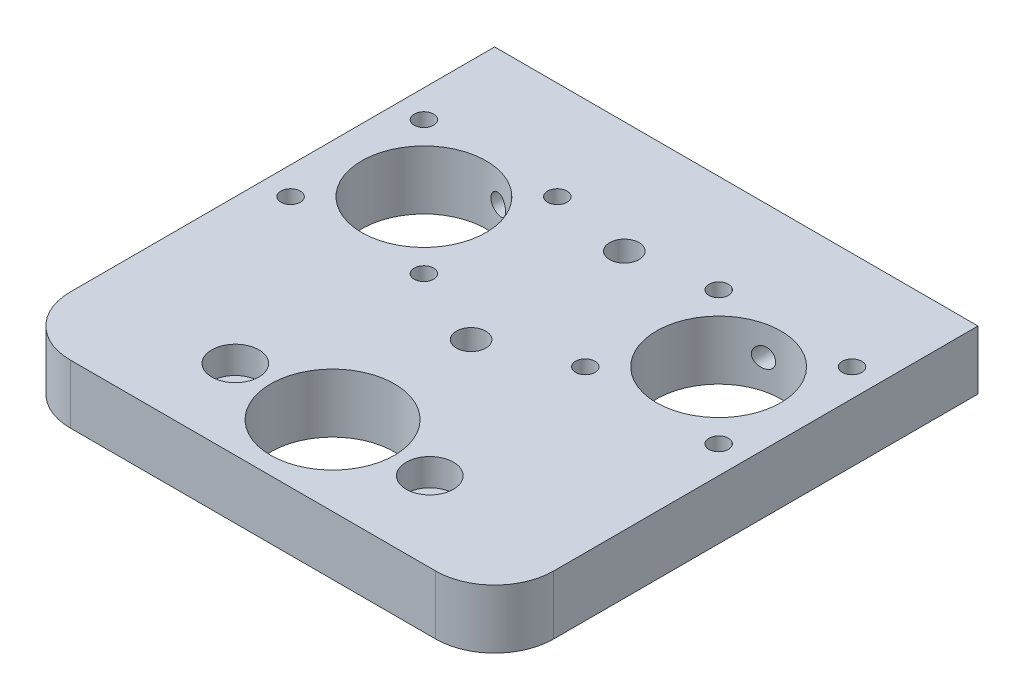
from build123d import *

# Parameters (mm, degrees)
SKETCH_1_W                = 82
SKETCH_1_H                = 82
EXTRUDE_1_DEPTH           = 10
SKETCH_4_R                = 10.5
CUT_EXTRUDE_3_DEPTH       = 59.838762733
FILLET_9_R                = 10
HOLE_WIZARD_2_D           = 4.3
HOLE_WIZARD_2_CBORE_D     = 8
HOLE_WIZARD_2_CBORE_DEPTH = 4.6
HOLE_WIZARD_M4_2_D        = 3.3
HOLE_WIZARD_M4_2_DEPTH    = 18.5
HOLE_WIZARD_M4_2_TIP      = 0.991420021
MM_2_D                    = 21.1
HOLE_WIZARD_M4_3_D        = 3.3
HOLE_WIZARD_M6_1_D        = 5
HOLE_WIZARD_M6_2_D        = 5
HOLE_WIZARD_5_0_5_1_D     = 5
HOLE_WIZARD_5_0_5_1_DEPTH = 10
HOLE_WIZARD_5_0_5_1_TIP   = 1.502151548


with BuildPart() as part:
    # 草图1 → 凸台-拉伸1 (new body)
    with BuildSketch(Plane(origin=(0, 0, 0), x_dir=(1, 0, 0), z_dir=(0, 1, 0))):
        Rectangle(SKETCH_1_W, SKETCH_1_H)
    extrude(amount=EXTRUDE_1_DEPTH)

    # 草图4 → 切除-拉伸3 (cut, through all)
    with BuildSketch(Plane(origin=(0, 10, 0), x_dir=(1, 0, 0), z_dir=(0, 1, 0))):
        with Locations(Location((0, -27.5, 0), (0, 0, 270))):
            Circle(SKETCH_4_R)
    extrude(amount=-CUT_EXTRUDE_3_DEPTH, mode=Mode.SUBTRACT)

    # 圆角9
    fillet_9_edges = [part.edges().sort_by_distance(p)[0] for p in [
        (41, 5, 41),
        (-41, 5, 41),
    ]]
    fillet(fillet_9_edges, radius=FILLET_9_R)

    # 打孔尺寸(%根据)开槽圆柱头螺钉的类型2 (through all)
    with Locations(Plane(origin=(0, 10, 0), x_dir=(1, 0, 0), z_dir=(0, 1, 0))):
        with Locations((-16.5, -27.5), (16.5, -27.5)):
            CounterBoreHole(HOLE_WIZARD_2_D / 2, HOLE_WIZARD_2_CBORE_D / 2, HOLE_WIZARD_2_CBORE_DEPTH)

    # M4 螺纹孔2
    with Locations(Plane(origin=(0, 0, -41), x_dir=(-1, 0, 0), z_dir=(0, 0, -1))):
        with Locations((-22.5, 5), (22.5, 5)):
            Hole(HOLE_WIZARD_M4_2_D / 2, depth=HOLE_WIZARD_M4_2_DEPTH)
            with Locations((0, 0, -(HOLE_WIZARD_M4_2_DEPTH + HOLE_WIZARD_M4_2_TIP / 2))):  # 118° drill point
                Cone(0, HOLE_WIZARD_M4_2_D / 2, HOLE_WIZARD_M4_2_TIP, mode=Mode.SUBTRACT)

    # 大小mm 暗销孔2 (through all)
    with Locations(Plane(origin=(0, 10, 0), x_dir=(1, 0, 0), z_dir=(0, 1, 0))):
        with Locations((-25, 13), (25, 13)):
            Hole(MM_2_D / 2)

    # M4 螺纹孔3 (through all)
    with Locations(Plane(origin=(0, 0, 0), x_dir=(-1, 0, 0), z_dir=(0, -1, 0))):
        with Locations((-13.686291501, 24.313708499), (-13.686291501, 1.686291501), (-36.313708499, 1.686291501), (-36.313708499, 24.313708499)):
            hole_wizard_m4_3 = Hole(HOLE_WIZARD_M4_3_D / 2)

    # 镜向2: M4 螺纹孔3 across plane
    add(hole_wizard_m4_3.mirror(Plane(origin=(0, 0, 0), x_dir=(0, 0, 1), z_dir=(1, 0, 0))), mode=Mode.SUBTRACT)

    # M6 螺纹孔1 (through all)
    with Locations(Plane(origin=(0, 10, 0), x_dir=(1, 0, 0), z_dir=(0, 1, 0))):
        with Locations((0, 22)):
            Hole(HOLE_WIZARD_M6_1_D / 2)

    # M6 螺纹孔2 (through all)
    with Locations(Plane(origin=(0, 10, 0), x_dir=(1, 0, 0), z_dir=(0, 1, 0))):
        with Locations((0, -4)):
            Hole(HOLE_WIZARD_M6_2_D / 2)

    # Ø5.0 (5) 直径孔1
    with Locations(Plane(origin=(0, 0, -41), x_dir=(-1, 0, 0), z_dir=(0, 0, -1))):
        with Locations((-32.5, 5), (32.5, 5)):
            Hole(HOLE_WIZARD_5_0_5_1_D / 2, depth=HOLE_WIZARD_5_0_5_1_DEPTH)
            with Locations((0, 0, -(HOLE_WIZARD_5_0_5_1_DEPTH + HOLE_WIZARD_5_0_5_1_TIP / 2))):  # 118° drill point
                Cone(0, HOLE_WIZARD_5_0_5_1_D / 2, HOLE_WIZARD_5_0_5_1_TIP, mode=Mode.SUBTRACT)


solid = part.part
